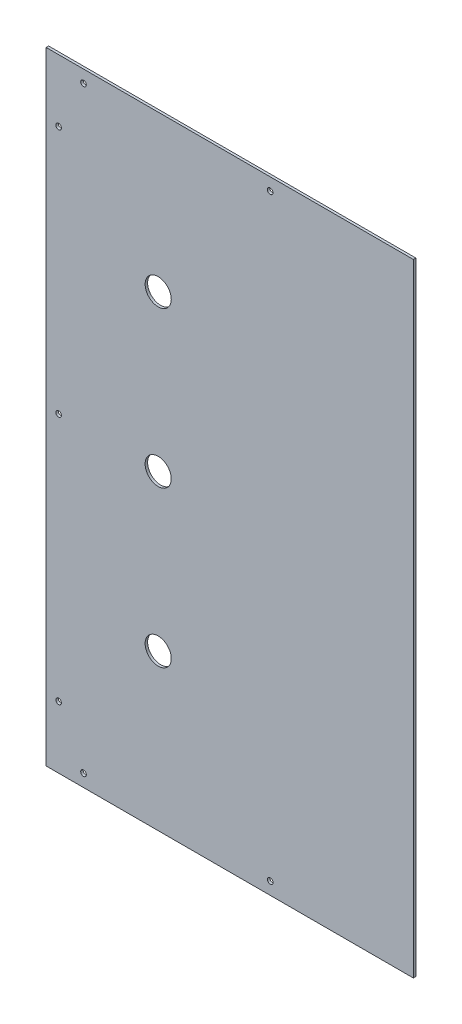
from build123d import *

# Parameters (mm, degrees)
SKETCH_1_W                  = 295
SKETCH_1_H                  = 500
EXTRUDE_1_DEPTH             = 2
HOLE_WIZARD_4_5_4_5_1_D     = 4.5
HOLE_WIZARD_4_5_4_5_1_DEPTH = 8
HOLE_WIZARD_4_5_4_5_1_TIP   = 1.351936393
SKETCH_4_R                  = 10.5
CUT_EXTRUDE_1_DEPTH         = 10


with BuildPart() as part:
    # 草图1 → 凸台-拉伸1 (new body)
    with BuildSketch(Plane.XY):
        Rectangle(SKETCH_1_W, SKETCH_1_H)
    extrude(amount=EXTRUDE_1_DEPTH)

    # Ø4.5 (4.5) 直径孔1
    with Locations(Plane.XY.offset(2)):
        with Locations((-117.5, -240), (-137.5, 0), (-137.5, 200), (-137.5, -200), (-117.5, 240), (32.5, 240), (32.5, -240)):
            Hole(HOLE_WIZARD_4_5_4_5_1_D / 2, depth=HOLE_WIZARD_4_5_4_5_1_DEPTH)
            with Locations((0, 0, -(HOLE_WIZARD_4_5_4_5_1_DEPTH + HOLE_WIZARD_4_5_4_5_1_TIP / 2))):  # 118° drill point
                Cone(0, HOLE_WIZARD_4_5_4_5_1_D / 2, HOLE_WIZARD_4_5_4_5_1_TIP, mode=Mode.SUBTRACT)

    # 草图4 → 切除-拉伸1 (cut)
    with BuildSketch(Plane.XY.offset(2)):
        with Locations((-57.5, 125)):
            Circle(SKETCH_4_R)
        with Locations((-57.5, -125)):
            Circle(SKETCH_4_R)
        with Locations((-57.5, 0)):
            Circle(SKETCH_4_R)
    extrude(amount=-CUT_EXTRUDE_1_DEPTH, mode=Mode.SUBTRACT)


solid = part.part
